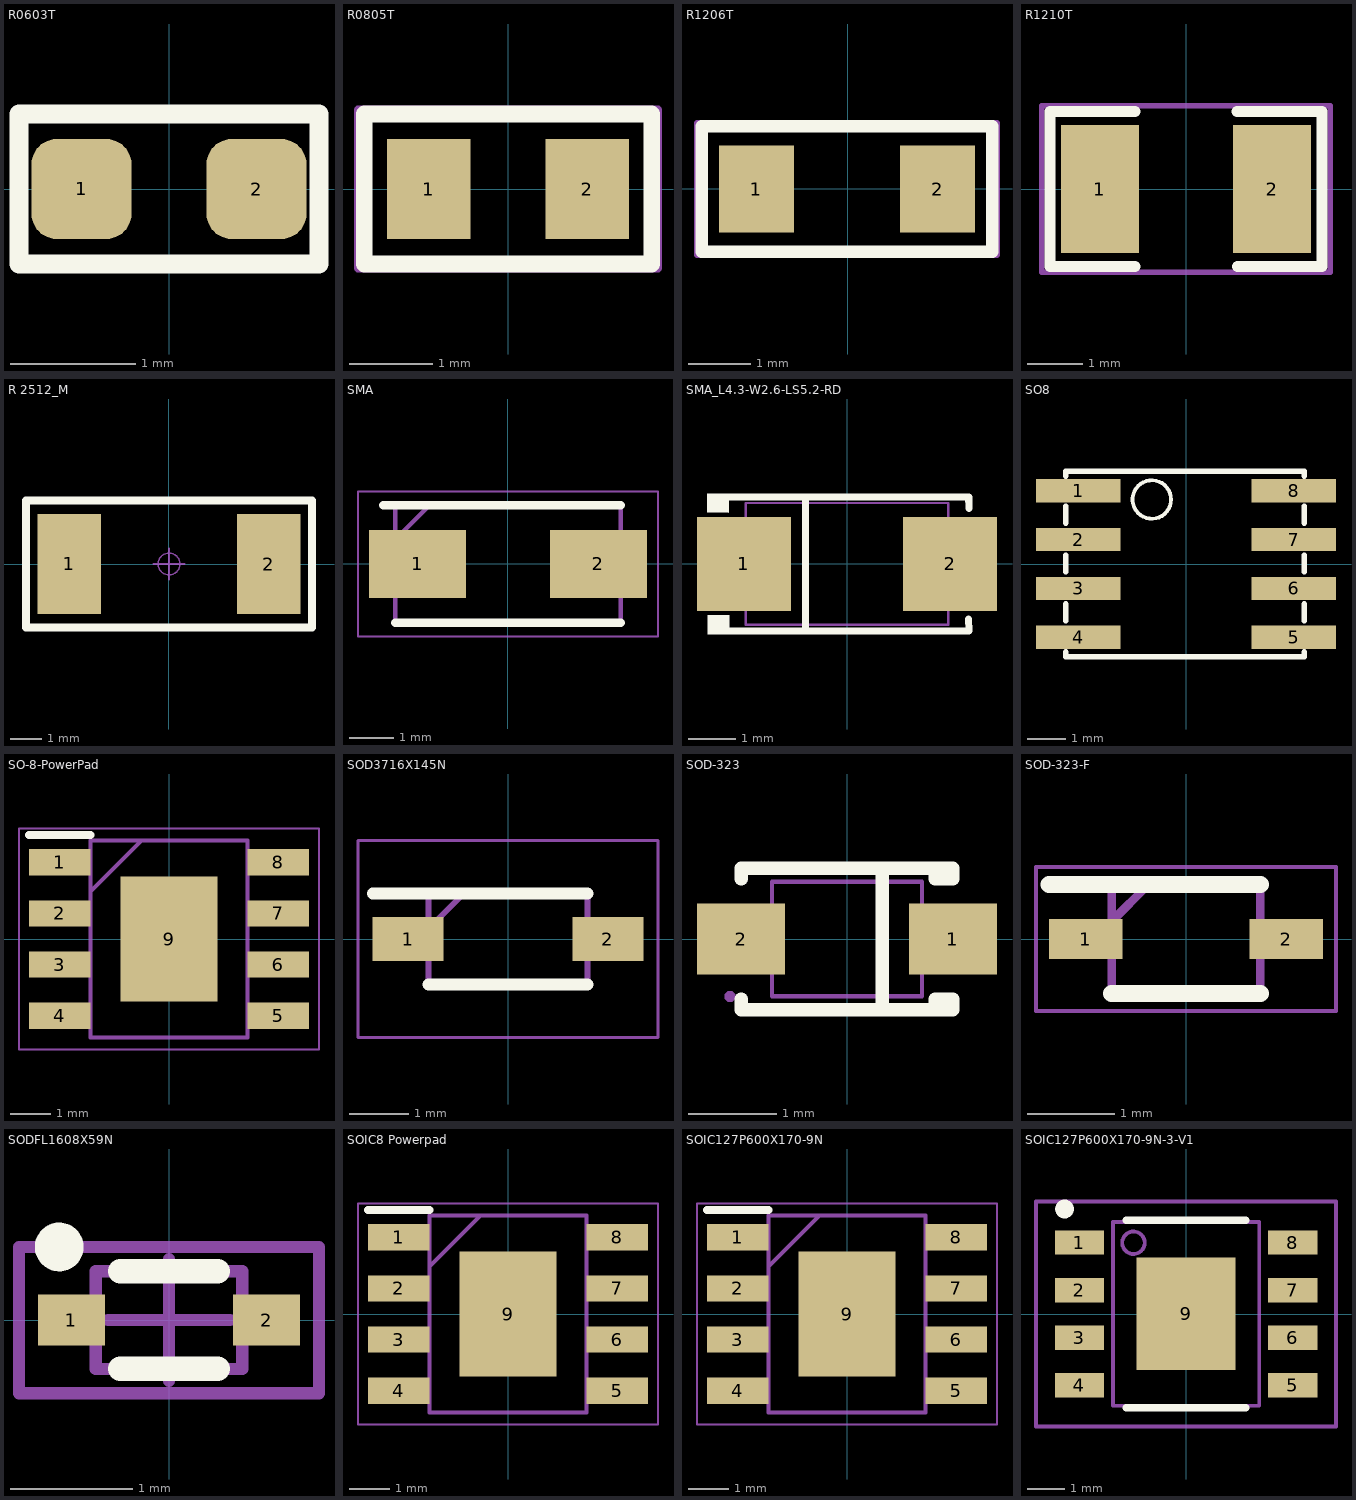
[diagram p0: the footprints below, top view; thin cyan lines are the x and y axes]
# Altium footprint library MISC82254-2.PcbLib: 93 footprints (part 4 of 6)
Each footprint in its own frame and in the unit in brackets; x right, y up, seen from the top. Pads: shape width x height; smd on the part's side, far side on the other; paste and mask are expansions set on the pad; w line width, h text height; cw(c..) or ccw(c..) is an arc to the next point about the centre after c.

## R0603T [mm]
height 1
pads (2):
  rrect50% 0.8x0.8 smd: 1(-0.7,0) 2(0.7,0)
Top Overlay:
  lines w0.15: -1.2,-0.6 1.2,-0.6 1.2,0.6 -1.2,0.6 -1.2,-0.6
3D body "R0603.step": height 0.8, standoff 0, extent -0.8,-0.406 0.8,0.394

## R0805T [mm]
pads (2):
  rect 1x1.2 smd: 1(-0.95,0) 2(0.95,0)
Top Overlay:
  lines w0.2: -1.725,-0.9 -1.725,0.9 1.725,0.9 1.725,-0.9 -1.725,-0.9
Mechanical 15:
  lines w0.1: -1.8,-0.95 -1.8,0.95 1.8,0.95 1.8,-0.95 -1.8,-0.95
3D body "CRGH0805F49K9.stp": height 0.65, standoff 0, extent -1,-0.637 1,0.637

## R1206T [mm]
pads (2):
  rect 1.2x1.4 smd: 1(-1.459,-0.006) 2(1.441,-0.006)
Top Overlay:
  lines w0.2: -2.334,-1.006 2.316,-1.006 2.316,0.994 -2.334,0.994 -2.334,-1.006
Mechanical 15:
  lines w0.1: -2.409,-1.056 2.391,-1.056 2.391,1.044 -2.409,1.044 -2.409,-1.056
3D body "CRGH1206J2M0.stp": height 0.65, standoff 0, extent -1.55,-0.787 1.55,0.787

## R1210T [mm]
pads (2):
  rect 1.4x2.3 smd: 1(-1.55,0) 2(1.55,0)
Top Overlay:
  lines w0.2: -0.915,-1.393 -2.45,-1.393 -2.45,1.393 -0.915,1.393 ; 0.915,1.393 2.45,1.393 2.45,-1.393 0.925,-1.393
Mechanical 15:
  lines w0.1: -2.6,-1.5 2.6,-1.5 2.6,1.5 -2.6,1.5 -2.6,-1.5
3D body "12105E103MAT2A.stp": height 0.94, standoff 0, extent -1.538,-1.263 1.662,1.237
3D body "CRCW12101R82FNEA.stp": height 0.6, standoff 0, extent -1.6,-1.25 1.6,1.25

## R 2512_M [mm] "1W贴片电阻"
pads (2):
  rect 2.032x3.2 smd: 1(-3.2,0) 2(3.2,0)
Top Overlay:
  lines w0.254: -4.572,-2.032 -4.572,2.032 4.572,2.032 4.572,-2.032 -4.572,-2.032
Mechanical 15:
  circle w0.05: c0,0 r0.35
  lines w0.05: -0.5,0 0.5,0 ; 0,-0.5 0,0.5
3D body "R 2512.STEP": height 0.55, standoff -0.02, extent -3.2,-1.6 3.2,1.6

## SMA [mm]
pads (2):
  rect 2.2x1.55 smd: 1(-2.05,0) 2(2.05,0)
Top Overlay:
  lines w0.2: -2.825,1.332 2.552,1.332 ; -2.552,-1.332 2.552,-1.332
Mechanical 13:
  lines w0.1: -2.552,0.558 -1.778,1.332 ; -2.552,-1.332 2.552,-1.332 2.552,1.332 -2.552,1.332 -2.552,-1.332
Mechanical 15:
  lines w0.05: -3.4,-1.645 3.4,-1.645 3.4,1.645 -3.4,1.645 -3.4,-1.645
3D body "VS-E7MH0112-M3_I.stp": height 2.25, standoff 0, extent -2.698,-1.778 2.702,1.778

## SMA_L4.3-W2.6-LS5.2-RD [mm]
pads (2):
  rect 2x2 smd: 1(-2.2,0) 2(2.2,0)
Top Overlay:
  region: -2.512,-1.096 -2.513,-1.503 -2.973,-1.498 -2.969,-1.096
  region: -2.52,1.502 -2.521,1.096 -2.981,1.1 -2.977,1.502
  lines w0.152: -2.596,-1.426 2.596,-1.426 ; -2.596,1.426 2.596,1.426 2.603,1.187 ; -0.884,-1.426 -0.884,1.426 ; 2.593,-1.176 2.6,-1.415
Mechanical 6:
  region: 2.014,-0.675 2.014,0.675 1.811,0.675 1.811,-0.675
  region: 2.29,-0.09 2.29,0.112 1.48,0.112 1.48,-0.09
  region: -2.317,-0.101 -2.317,0.101 -1.507,0.101 -1.507,-0.101
Mechanical 15:
  region: -1.48,0.725 -1.48,-0.725 -2.605,-0.725 -2.605,0.725
  region: 2.605,0.725 2.605,-0.725 1.48,-0.725 1.48,0.725
  region: -2.545,-1.3 -2.546,-1.275 -2.58,-1.241 -2.629,-1.241 -2.664,-1.275 -2.665,-1.3 -2.664,-1.324 -2.63,-1.359 -2.581,-1.359 -2.546,-1.324
  lines w0.051: -2.16,-1.3 2.16,-1.3 2.16,1.3 -2.16,1.3 -2.16,-1.3
3D body "VS-E7MH0112-M3_I.stp": height 2.25, standoff 0, extent -2.698,-1.778 2.702,1.778

## SO8 [mm]
height 2.55
pads (8):
  rect 2.2x0.6 smd: 1(-2.8,1.905) 2(-2.8,0.635) 3(-2.8,-0.635) 4(-2.8,-1.905) 5(2.8,-1.905) 6(2.8,-0.635) 7(2.8,0.635) 8(2.8,1.905)
Top Overlay:
  circle w0.1: c-0.889,1.676 r0.5
  lines w0.15: -3.124,-2.286 -3.124,-2.413 3.073,-2.413 3.073,-2.286 ; -3.124,-1.473 -3.124,-1.041 ; -3.124,-0.203 -3.124,0.229 ; -3.124,1.067 -3.124,1.499 ; -3.124,2.286 -3.124,2.413 3.073,2.413 3.073,2.286 ; 3.073,-1.473 3.073,-1.041 ; 3.073,-0.203 3.073,0.229 ; 3.073,1.067 3.073,1.499
3D body "SOIC8.step": height 1.76, standoff 0, extent -3.1,-2.402 3.1,2.398

## SO-8-PowerPad [mm]
pads (9):
  rect 1.525x0.65 smd: 1(-2.712,1.905) 2(-2.712,0.635) 3(-2.712,-0.635) 4(-2.712,-1.905) 5(2.712,-1.905) 6(2.712,-0.635) 7(2.712,0.635) 8(2.712,1.905)
  rect 2.4x3.1 smd: 9(0,0)
Top Overlay:
  lines w0.2: -3.475,2.58 -1.95,2.58
Mechanical 13:
  lines w0.1: -1.95,1.18 -0.68,2.45 ; -1.95,-2.45 1.95,-2.45 1.95,2.45 -1.95,2.45 -1.95,-2.45
Mechanical 15:
  lines w0.05: -3.725,-2.75 3.725,-2.75 3.725,2.75 -3.725,2.75 -3.725,-2.75
3D body "UCC27210DDAR.stp": height 1.57, standoff 0, extent -3,-2.45 3,2.45

## SOD3716X145N [mm]
pads (2):
  rect 1.2x0.75 smd: 1(-1.7,0) 2(1.7,0)
Top Overlay:
  lines w0.2: -2.3,0.775 1.35,0.775 ; -1.35,-0.775 1.35,-0.775
Mechanical 13:
  lines w0.1: -1.35,0.175 -0.75,0.775 ; -1.35,-0.775 -1.35,0.775 1.35,0.775 1.35,-0.775 -1.35,-0.775
Mechanical 15:
  lines w0.05: -2.55,-1.675 -2.55,1.675 2.55,1.675 2.55,-1.675 -2.55,-1.675
3D body "MMSZ5231B-7-F.stp": height 1.45, standoff 0, extent -1.85,-0.775 1.85,0.775

## SOD-323 [mm]
pads (2):
  rect 1x0.8 smd: 1(1.2,0) 2(-1.2,0)
Top Overlay:
  lines w0.152: -1.2,-0.68 -1.2,-0.8 -1,-0.8 1,-0.8 ; -1.2,0.68 -1.2,0.8 -1,0.8 1,0.8 ; 0.4,-0.8 0.4,0.8 ; 1,-0.8 1.2,-0.8 1.2,-0.68 1,-0.68 1,-0.8 ; 1,0.8 1.2,0.8 1.2,0.68 1,0.68 1,0.8
Mechanical 6:
  region: 0.9,0.1 1.6,0.1 1.6,0 1.6,-0.1 0.9,-0.1
  region: -1.55,0.1 -0.85,0.1 -0.85,0 -0.85,-0.1 -1.55,-0.1
  region: -1.3,-0.35 -1.3,0.35 -1.2,0.35 -1.1,0.35 -1.1,-0.35
Mechanical 15:
  region: -1.265,-0.65 -1.265,-0.625 -1.3,-0.59 -1.35,-0.59 -1.385,-0.625 -1.385,-0.65 -1.385,-0.675 -1.35,-0.71 -1.3,-0.71 -1.265,-0.675
  region: -1.01,-0.15 -1.01,0.15 -0.84,0.15 -0.84,-0.15
  region: -1.325,-0.15 -1.325,0.15 -1,0.15 -1,-0.15
  region: 0.84,-0.15 0.84,0.15 1.01,0.15 1.01,-0.15
  region: 1,-0.15 1,0.15 1.325,0.15 1.325,-0.15
  lines w0.051: -0.85,-0.65 -0.85,0.65 0.85,0.65 0.85,-0.65 -0.85,-0.65
3D body "BAS316,115.stp": height 0.93, standoff 0, extent -1.245,-0.627 1.244,0.623

## SOD-323-F [mm]
pads (2):
  rect 0.84x0.46 smd: 1(-1.15,0) 2(1.15,0)
Top Overlay:
  lines w0.2: -1.57,0.625 0.85,0.625 ; -0.85,-0.625 0.85,-0.625
Mechanical 13:
  lines w0.1: -0.85,0.205 -0.43,0.625 ; -0.85,-0.625 0.85,-0.625 0.85,0.625 -0.85,0.625 -0.85,-0.625
Mechanical 15:
  lines w0.05: -1.72,-0.825 1.72,-0.825 1.72,0.825 -1.72,0.825 -1.72,-0.825
3D body "PMEG2010EJ,115.stp": height 0.71, standoff 0, extent -1.251,-0.627 1.249,0.623

## SODFL1608X59N [mm] "SODFL Diode;1.20mm W X 0.80mm L X 0.59mm H body"
height 0.59
pads (2):
  rect 0.55x0.42 smd paste+0 mask+0: 1(-0.8,0) 2(0.8,0)
Top Overlay:
  circle w0.2: c-0.9,0.6 r0.1
  lines w0.2: -0.4,-0.4 0.4,-0.4 ; -0.4,0.4 0.4,0.4
Mechanical 3:
  text ".DESIGNATOR" at 0,0 h1.2
Mechanical 13:
  lines w0.1: -0.6,-0.4 -0.6,0.4 0.6,0.4 0.6,-0.4 -0.6,-0.4
Mechanical 15:
  lines w0.1: -0.5,0 0.5,0 ; 0,-0.5 0,0.5 ; -1.23,-0.6 -1.23,0.6 1.23,0.6 1.23,-0.6 -1.23,-0.6
3D body "SC79-2-1.stp": height 0.59, standoff 0, extent -0.8,-0.4 0.8,0.4

## SOIC8 Powerpad [mm]
pads (9):
  rect 1.525x0.65 smd: 1(-2.712,1.905) 2(-2.712,0.635) 3(-2.712,-0.635) 4(-2.712,-1.905) 5(2.712,-1.905) 6(2.712,-0.635) 7(2.712,0.635) 8(2.712,1.905)
  rect 2.4x3.1 smd: 9(0,0)
Top Overlay:
  lines w0.2: -3.475,2.58 -1.95,2.58
Mechanical 13:
  lines w0.1: -1.95,1.18 -0.68,2.45 ; -1.95,-2.45 -1.95,2.45 1.95,2.45 1.95,-2.45 -1.95,-2.45
Mechanical 15:
  lines w0.05: -3.725,-2.75 -3.725,2.75 3.725,2.75 3.725,-2.75 -3.725,-2.75
3D body "UCC27210DDAR.stp": height 1.57, standoff 0, extent -3,-2.45 3,2.45

## SOIC127P600X170-9N [mm]
pads (9):
  rect 1.525x0.65 smd: 1(-2.712,1.905) 2(-2.712,0.635) 3(-2.712,-0.635) 4(-2.712,-1.905) 5(2.712,-1.905) 6(2.712,-0.635) 7(2.712,0.635) 8(2.712,1.905)
  rect 2.4x3.1 smd: 9(0,0)
Top Overlay:
  lines w0.2: -3.475,2.58 -1.95,2.58
Mechanical 13:
  lines w0.1: -1.95,1.18 -0.68,2.45 ; -1.95,-2.45 1.95,-2.45 1.95,2.45 -1.95,2.45 -1.95,-2.45
Mechanical 15:
  lines w0.05: -3.725,-2.75 3.725,-2.75 3.725,2.75 -3.725,2.75 -3.725,-2.75
3D body "UCC27210DDAR.stp": height 1.57, standoff 0, extent -3,-2.45 3,2.45

## SOIC127P600X170-9N-3-V1 [mm] "SOIC,1.27mm pitch;8 pin,3.90mm W X 4.90mm L X 1.70mm H body (w/thermal tab)"
height 1.7
pads (9):
  rect 1.31x0.65 smd paste+0 mask+0: 1(-2.845,1.905) 2(-2.845,0.635) 3(-2.845,-0.635) 4(-2.845,-1.905) 5(2.845,-1.905) 6(2.845,-0.635) 7(2.845,0.635) 8(2.845,1.905)
  rect 2.65x3 smd paste-1.5 mask+0: 9(0,0)
Top Overlay:
  circle w0.25: c-3.24,2.8 r0.125
  lines w0.2: -1.6,-2.5 1.6,-2.5 ; -1.6,2.5 1.6,2.5
Top Paste:
  region: 0.2,-0.2 1.225,-0.2 1.225,-1.4 0.2,-1.4
  region: 0.2,-0.2 1.225,-0.2 1.225,-1.4 0.2,-1.4
  region: -0.2,0.2 -1.225,0.2 -1.225,1.4 -0.2,1.4
  region: -0.2,-0.2 -1.225,-0.2 -1.225,-1.4 -0.2,-1.4
  region: 0.2,0.2 1.225,0.2 1.225,1.4 0.2,1.4
Mechanical 3:
  text ".DESIGNATOR" at 0,0 h1.2
Mechanical 13:
  circle w0.1: c-1.4,1.9 r0.3
  lines w0.1: -1.95,-2.45 1.95,-2.45 1.95,2.45 -1.95,2.45 -1.95,-2.45
Mechanical 15:
  lines w0.1: -0.5,0 0.5,0 ; 0,-0.5 0,0.5 ; -4,-3 -4,3 4,3 4,-3 -4,-3
3D body "PG-DSO-8-52.STEP": height 1.71, standoff 0, extent -3,-2.45 3,2.45